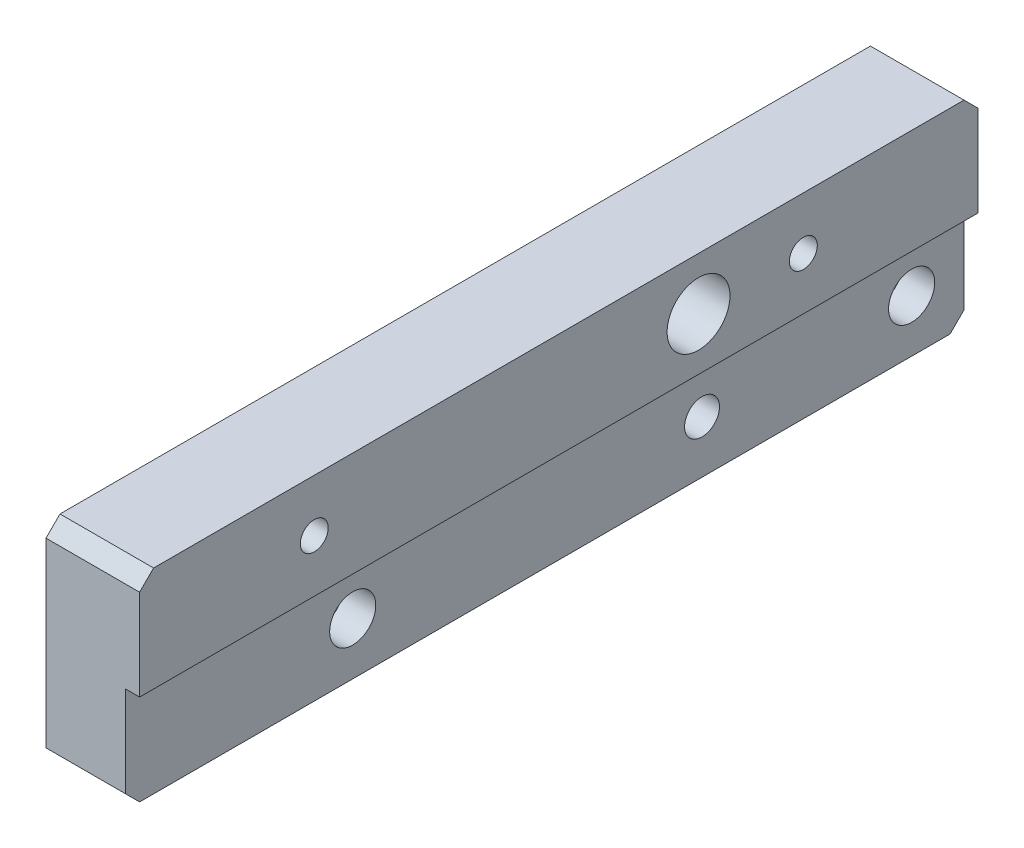
from build123d import *

# Parameters (mm, degrees)
SKETCH1_W                                            = 120
SKETCH1_H                                            = 30
BOSS_EXTRUDE1_DEPTH                                  = 13.4
SKETCH2_W                                            = 120
SKETCH2_H                                            = 15
CUT_EXTRUDE1_DEPTH                                   = 2
HOLE1_AT_2_COUNT                                     = 2
HOLE1_AT_2_PITCH                                     = 70
M8_CLEARANCE_HOLE1_D                                 = 9
CHAMFER1_SIZE                                        = 2
CBORE_FOR_M6_HEXAGON_SOCKET_HEAD_CAP_SCR_D           = 6.6
CBORE_FOR_M6_HEXAGON_SOCKET_HEAD_CAP_SCR_CBORE_D     = 11
CBORE_FOR_M6_HEXAGON_SOCKET_HEAD_CAP_SCR_CBORE_DEPTH = 6.8
F_5_0MM_BLIND_HOLE_1_D                               = 5


with BuildPart() as part:
    # Sketch1 → Boss-Extrude1 (new body)
    with BuildSketch(Plane(origin=(0, 0, 0), x_dir=(0, 0, -1), z_dir=(1, 0, 0))):
        Rectangle(SKETCH1_W, SKETCH1_H)
    extrude(amount=BOSS_EXTRUDE1_DEPTH)

    # Sketch2 → Cut-Extrude1 (cut)
    with BuildSketch(Plane(origin=(13.4, 0, 0), x_dir=(0, 0, -1), z_dir=(1, 0, 0))):
        with Locations((0, -7.5)):
            Rectangle(SKETCH2_W, SKETCH2_H)
    extrude(amount=-CUT_EXTRUDE1_DEPTH, mode=Mode.SUBTRACT)

    # Sketch4 → Hole1 (revolve, cut)
    with BuildSketch(Plane(origin=(0, 7.5, 35), x_dir=(0, 0, 1), z_dir=(0, 1, 0))):
        Polygon((0, 0), (0, 20), (2, 20), (2, 8.701721238), (4, 7.5), (4, 0), align=None)
    hole1 = revolve(axis=Axis((-6.130023899, 7.5, 35), (1, 0, 0)), mode=Mode.SUBTRACT)

    # Hole1 at 2: Hole1 ×2
    with Locations(*[(0, 0, -i * HOLE1_AT_2_PITCH) for i in range(1, HOLE1_AT_2_COUNT)]):
        add(hole1, mode=Mode.SUBTRACT)

    # M8 Clearance Hole1 (through all)
    with Locations(Plane(origin=(13.4, 0, 0), x_dir=(0, 0, -1), z_dir=(1, 0, 0))):
        with Locations((20, 7.5)):
            Hole(M8_CLEARANCE_HOLE1_D / 2)

    # Chamfer1
    chamfer1_edges = [part.edges().sort_by_distance(p)[0] for p in [
        (5.7, -15, -60),
        (5.7, -15, 60),
        (6.7, 15, 60),
        (6.7, 15, -60),
    ]]
    chamfer(chamfer1_edges, length=CHAMFER1_SIZE)

    # CBORE for M6 Hexagon socket head cap screws1 (through all)
    with Locations(Plane.ZY):
        with Locations((-52.5, -7.5), (27.5, -7.5)):
            CounterBoreHole(CBORE_FOR_M6_HEXAGON_SOCKET_HEAD_CAP_SCR_D / 2, CBORE_FOR_M6_HEXAGON_SOCKET_HEAD_CAP_SCR_CBORE_D / 2, CBORE_FOR_M6_HEXAGON_SOCKET_HEAD_CAP_SCR_CBORE_DEPTH)

    # Ø5.0mm blind hole 1 (through all)
    with Locations(Plane.ZY):
        with Locations((-22.5, -7.5)):
            Hole(F_5_0MM_BLIND_HOLE_1_D / 2)


solid = part.part
